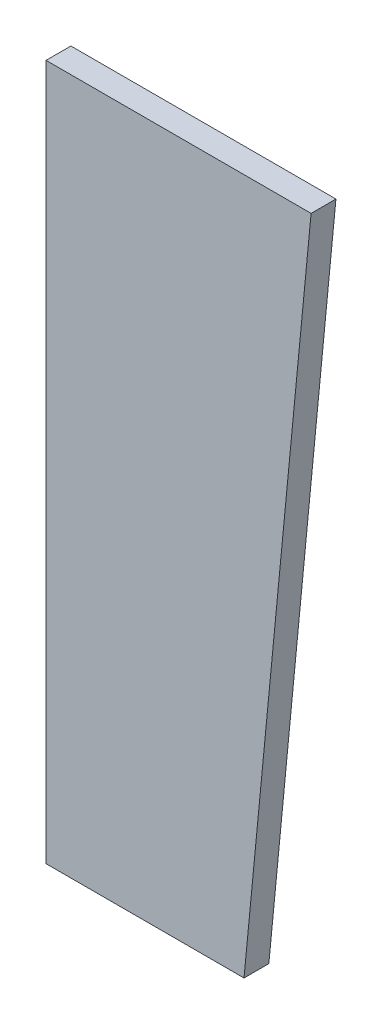
SolidWorks part; units mm, degrees
material "Q235B"
ref_plane "Front Plane" through (0, 0, 0) normal (0, 0, 1) x (1, 0, 0)
ref_plane "Top Plane" through (0, 0, 0) normal (0, 1, 0) x (1, 0, 0)
ref_plane "Right Plane" through (0, 0, 0) normal (1, 0, 0) x (0, 0, -1)
sketch "Sketch1" plane through (0, 0, 0) normal (0, 0, 1) x (1, 0, 0)
  line L0 (0, 0) -> (239, 0)
  line L1 (239, 0) -> (320, 840)
  line L2 (320, 840) -> (0, 840)
  line L3 (0, 840) -> (0, 0)
  dimension "D1" = 239
  dimension "D2" = 320
  dimension "D3" = 840
extrude "Boss-Extrude1" add sketch "Sketch1" along normal blind 30
